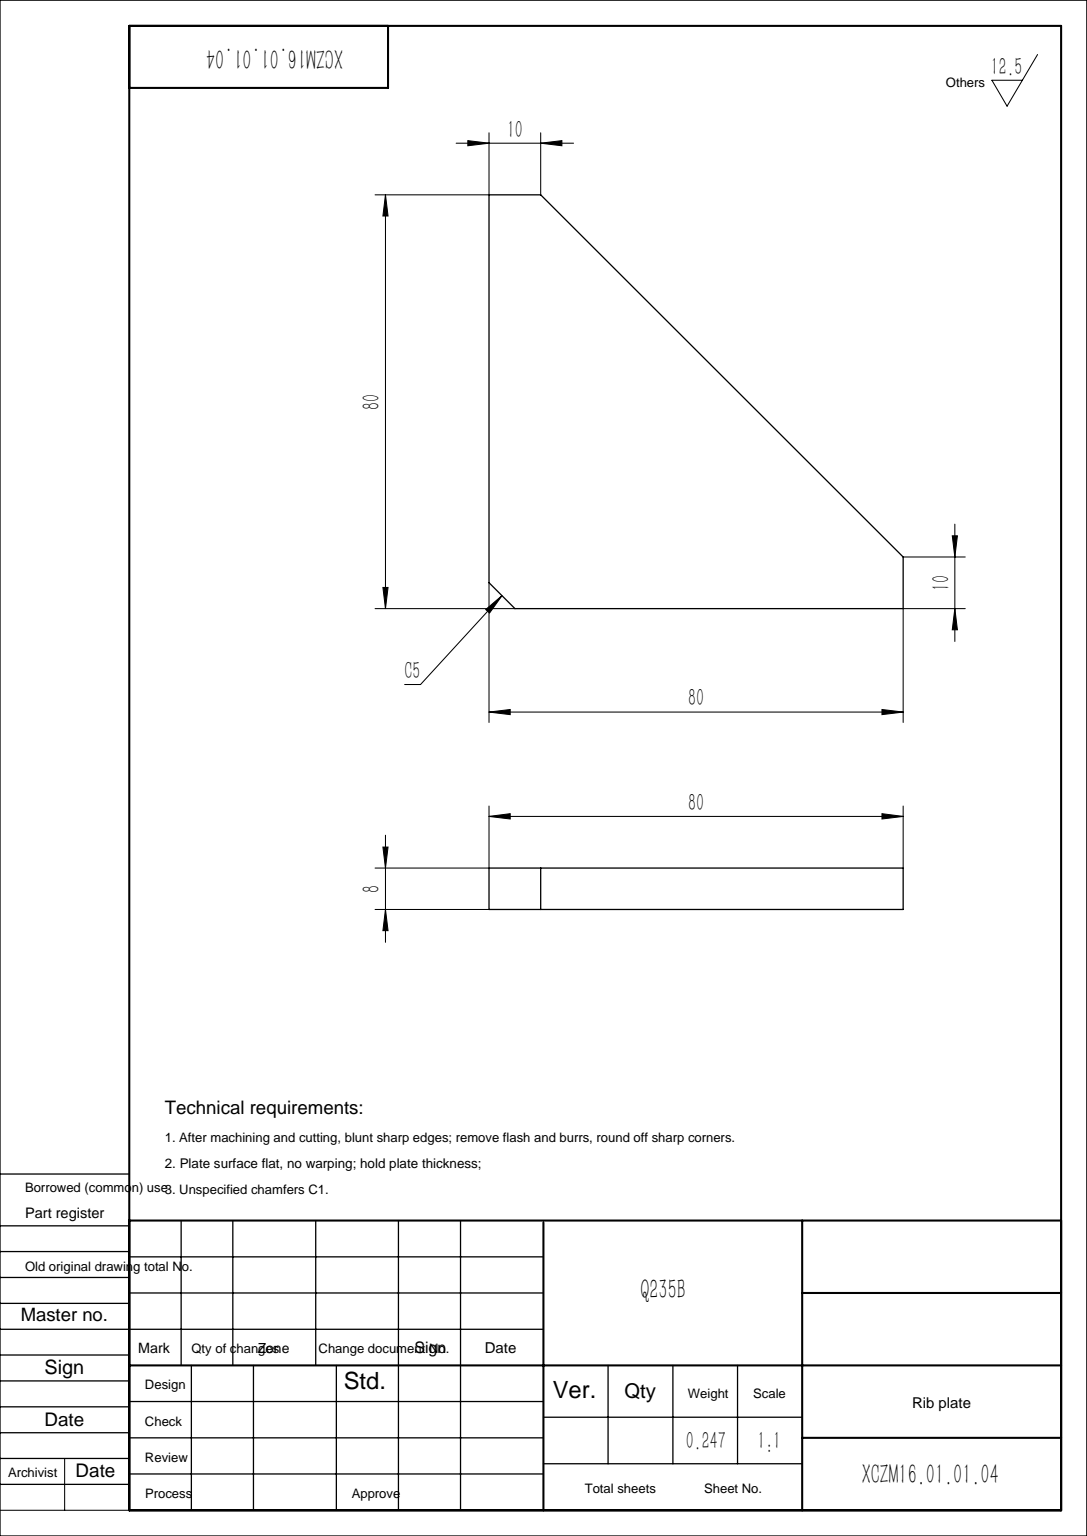
from build123d import *

# Parameters (mm, degrees)
BOSS_EXTRUDE1_DEPTH = 8
CHAMFER1_SIZE       = 5


with BuildPart() as part:
    # Sketch1 → Boss-Extrude1 (new body)
    with BuildSketch(Plane.XY):
        Polygon((0, 80), (0, 0), (80, 0), (80, 10), (10, 80), align=None)
    extrude(amount=BOSS_EXTRUDE1_DEPTH)

    # Chamfer1
    chamfer1_edges = [part.edges().sort_by_distance(p)[0] for p in [
        (0, 0, 4),
    ]]
    chamfer(chamfer1_edges, length=CHAMFER1_SIZE)


solid = part.part
